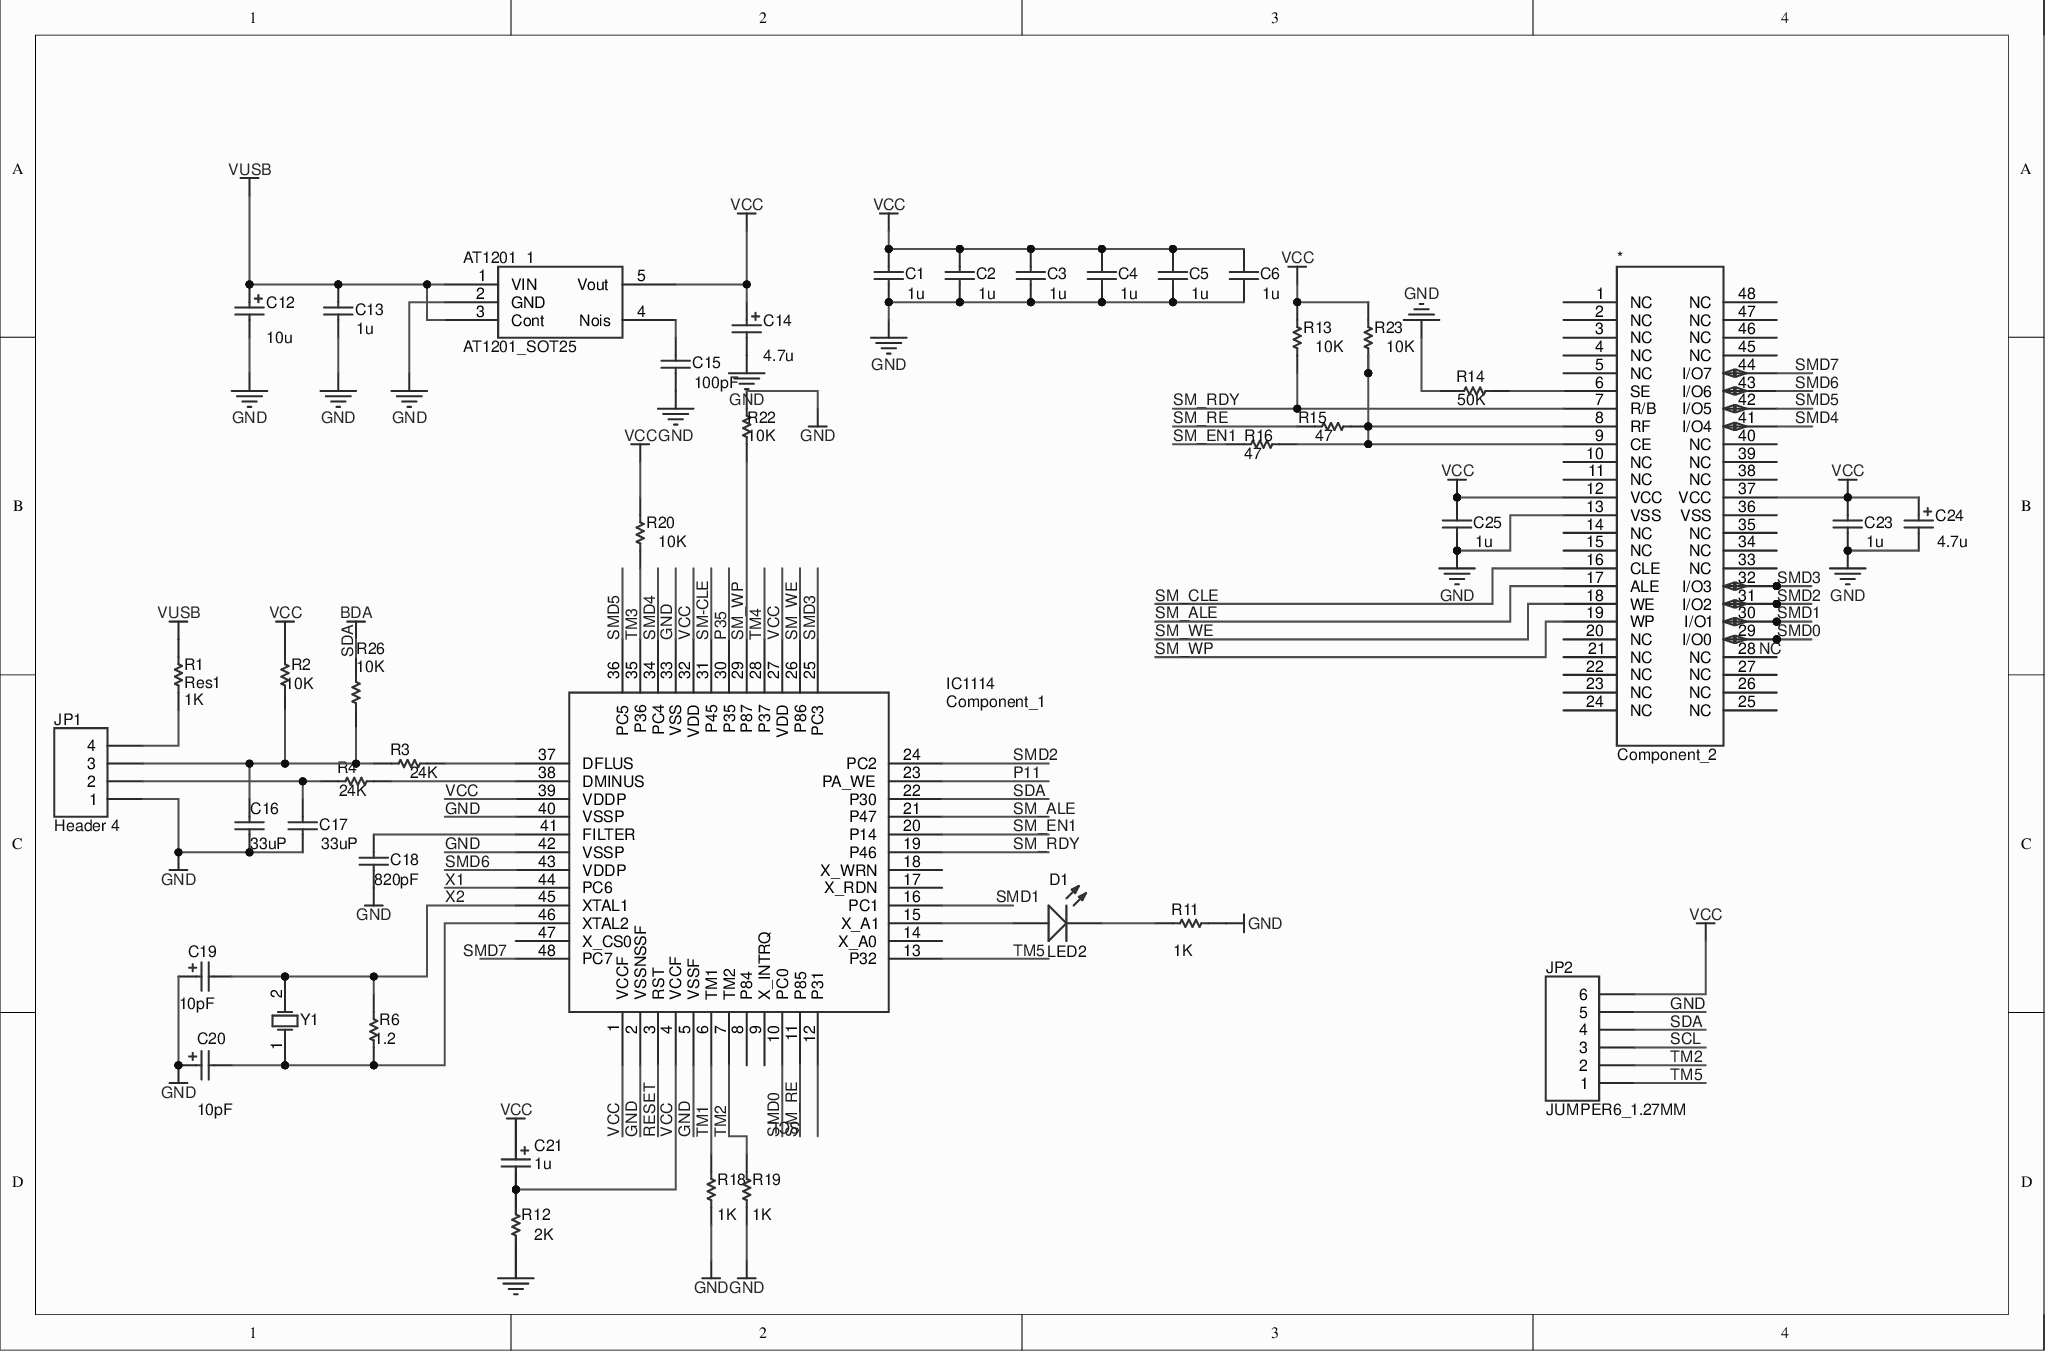
[diagram p0: MISC75231-3.schdoc]
# Altium project MISC75231-2.PrjPcb
1 sheet, 43 parts. Net scope: global (net labels, ports and power ports of the same name join across sheets).
Board file: MISC75231.pcbdoc

## Sheet MISC75231-3.schdoc
size 292 x 193 mm; Name: MISC75231

### Parts
*  Component_2  [DIP48]
AT1201_1  AT1201_SOT25  [SOP6]
C1  value 1u  [RAD-0.3]
C2  value 1u  [RAD-0.3]
C3  value 1u  [RAD-0.3]
C4  value 1u  [RAD-0.3]
C5  value 1u  [RAD-0.3]
C6  value 1u  [RAD-0.3]
C12  value 10u  [POLAR0.8]
C13  value 1u  [RAD-0.3]
C14  value 4.7u  [POLAR0.8]
C15  value 100pF  [RAD-0.3]
C16  value 33uP  [RAD-0.3]
C17  value 33uP  [RAD-0.3]
C18  value 820pF  [RAD-0.3]
C19  value 10pF  [POLAR0.8]
C20  value 10pF  [POLAR0.8]
C21  value 1u  [POLAR0.8]
C23  value 1u  [RAD-0.3]
C24  value 4.7u  [POLAR0.8]
C25  value 1u  [RAD-0.3]
D1  LED2  [3.2X1.6X1.1]
IC1114  Component_1  [Quad48]
JP1  Header 4  [HDR1X4]
JP2  JUMPER6_1.27MM  [HDR1X6]
R1  Res1  value 1K  [AXIAL-0.3]
R2  value 10K  [AXIAL-0.3]
R3  value 24K  [AXIAL-0.3]
R4  value 24K  [AXIAL-0.3]
R6  value 1.2  [AXIAL-0.3]
R11  value 1K  [AXIAL-0.3]
R12  value 2K  [AXIAL-0.3]
R13  value 10K  [AXIAL-0.3]
R14  value 50K  [AXIAL-0.3]
R15  value 47  [AXIAL-0.3]
R16  value 47  [AXIAL-0.3]
R18  value 1K  [AXIAL-0.3]
R19  value 1K  [AXIAL-0.3]
R20  value 10K  [AXIAL-0.3]
R22  value 10K  [AXIAL-0.3]
R23  value 10K  [AXIAL-0.3]
R26  value 10K  [AXIAL-0.3]
Y1  (no value)  [R38]

### Nets
GND: *.13(VSS) AT1201_1.2(GND) C1.1 C2.1 C3.1 C4.1 C5.1 C6.1 C12.2 C13.1 C14.2 C15.1 C16.1 C17.2 C18.1 C19.1 C20.1 C23.1 C24.2 C25.1 IC1114.2(VSSNSSF) IC1114.5(VSSF) IC1114.33(VSS) IC1114.40(VSSP) IC1114.42(VSSP) JP1.1 JP2.5 R11.2 R12.1 R14.2 R18.1 R19.1 R22.2
BDA: IC1114.22(P30) JP2.4 R26.2  [also labelled SDA]
VCC: *.12(VCC) *.37(VCC) AT1201_1.5(Vout) C1.2 C2.2 C3.2 C4.2 C5.2 C6.2 C14.1 C21.1 C21.2 C23.2 C24.1 C25.2 IC1114.1(VCCF) IC1114.4(VCCF) IC1114.27(VDD) IC1114.32(VDD) IC1114.39(VDDP) JP2.6 R2.2 R12.2 R13.2 R20.2 R23.2
VUSB: AT1201_1.1(VIN) AT1201_1.3(Cont) C12.1 C13.2 R1.2
P11: IC1114.23(PA_WE)
P35: IC1114.30(P35)
RESET: IC1114.3(RST)
SCL: IC1114.11(P85) JP2.3 R15.1  [also labelled SM_RE]
SM-CLE: IC1114.31(P45)
SM_ALE: *.17(ALE) IC1114.21(P47)
SM_CLE: *.16(CLE)
SM_EN1: IC1114.20(P14) R16.1
SM_RDY: *.7(R/B) IC1114.19(P46) R13.1
SM_WE: *.18(WE) IC1114.26(P86)
SM_WP: *.19(WP) IC1114.29(P87) R22.1
SMD0: *.29(I/O0) IC1114.10(PC0)
SMD1: *.30(I/O1) IC1114.16(PC1)
SMD2: *.31(I/O2) IC1114.24(PC2)
SMD3: *.32(I/O3) IC1114.25(PC3)
SMD4: *.41(I/O4) IC1114.34(PC4)
SMD5: *.42(I/O5) IC1114.36(PC5)
SMD6: *.43(I/O6) IC1114.43(VDDP)
SMD7: *.44(I/O7)
TM1: IC1114.6(TM1) R18.2
TM2: IC1114.7(TM2) JP2.2 R19.2
TM3: IC1114.35(P36) R20.1
TM4: IC1114.28(P37)
TM5: IC1114.13(P32) JP2.1
X1: IC1114.44(PC6)
X2: C19.2 IC1114.45(XTAL1) R6.2 Y1.2(OSC2)
Net*_6: *.6(SE) R14.1
Net*_8: *.8(RF) *.9(CE) R15.2 R16.2 R23.1
NetAT1201_1_4: AT1201_1.4(Nois) C15.2
NetC16_2: C16.2 JP1.3 R2.1 R3.1 R26.1
NetC17_1: C17.1 JP1.2 R4.1
NetC18_2: C18.2 IC1114.41(FILTER)
NetC20_2: C20.2 IC1114.46(XTAL2) R6.1 Y1.1(OSC1)
NetD1_1: D1.1(A) IC1114.15(X_A1)
NetD1_2: D1.2(K) R11.1
NetIC1114_37: IC1114.37(DFLUS) R3.2
NetIC1114_38: IC1114.38(DMINUS) R4.2
NetJP1_4: JP1.4 R1.1

Not connected (* = marked no-connect by the designer): * 1(NC)* 2(NC)* 3(NC)* 4(NC)* 5(NC)* 10(NC)* 11(NC)* 14(NC) 15(NC)* 20(NC)* 21(NC)* 22(NC)* 23(NC)* 24(NC)* 25(NC)* 26(NC)* 27(NC)* 28(NC)* 33(NC)* 34(NC)* 35(NC)* 36(VSS) 38(NC)* 39(NC)* 40(NC)* 45(NC)* 46(NC)* 47(NC)* 48(NC)*; IC1114 8(P84)* 9(X_INTRQ)* 12(P31) 14(X_A0) 17(X_RDN)* 18(X_WRN)* 47(X_CS0)* 48(PC7)

### Notes on the sheet
- Labels drawn without touching a wire or pin: NC, SMD7

### Library data of the parts
* = Component_2: UniqueId: dc55b09e814ab7ff; AddInBom: yes; Device: Component_2; DesignItemID: Component_2; LibraryName: Schlib1; SymbolName: Component_2; FootprintName: DIP48
AT1201_1 = AT1201_SOT25: UniqueId: a1da92f836eef546; SymbolName: Component_3; AddInBom: yes; Device: AT1201_SOT25; DesignItemID: Component_3; LibraryName: Schlib1; FootprintName: SOP6
C1 = C1: Capacitor; UniqueId: 5fb4f22ffcb6a001; SymbolName: Cap; AddInBom: yes; Device: C1; Published: 8-Jun-2000; LatestRevisionDate: 17-Jul-2002; LatestRevisionNote: Re-released for DXP Platform.; PackageReference: RAD-0.3; PackageDescription: Radial Cap, Thru-Hole; 2 Leads; 0.3 in Pin Spacing; DesignItemID: Cap; LibraryName: Miscellaneous Devices; FootprintName: RAD-0.3; Publisher: Altium Limited
C2 = C2: Capacitor; UniqueId: 21d50210554cb61f; SymbolName: Cap; AddInBom: yes; Device: C2; Published: 8-Jun-2000; LatestRevisionDate: 17-Jul-2002; LatestRevisionNote: Re-released for DXP Platform.; PackageReference: RAD-0.3; PackageDescription: Radial Cap, Thru-Hole; 2 Leads; 0.3 in Pin Spacing; DesignItemID: Cap; LibraryName: Miscellaneous Devices; FootprintName: RAD-0.3; Publisher: Altium Limited
C3 = C3: Capacitor; UniqueId: ec64484c8c07847f; SymbolName: Cap; AddInBom: yes; Device: C3; Published: 8-Jun-2000; LatestRevisionDate: 17-Jul-2002; LatestRevisionNote: Re-released for DXP Platform.; PackageReference: RAD-0.3; PackageDescription: Radial Cap, Thru-Hole; 2 Leads; 0.3 in Pin Spacing; DesignItemID: Cap; LibraryName: Miscellaneous Devices; FootprintName: RAD-0.3; Publisher: Altium Limited
C4 = C4: Capacitor; UniqueId: 623e2bb2442f04df; SymbolName: Cap; AddInBom: yes; Device: C4; Published: 8-Jun-2000; LatestRevisionDate: 17-Jul-2002; LatestRevisionNote: Re-released for DXP Platform.; PackageReference: RAD-0.3; PackageDescription: Radial Cap, Thru-Hole; 2 Leads; 0.3 in Pin Spacing; DesignItemID: Cap; LibraryName: Miscellaneous Devices; FootprintName: RAD-0.3; Publisher: Altium Limited
C5 = C5: Capacitor; UniqueId: 05d417a4d81547fc; SymbolName: Cap; AddInBom: yes; Device: C5; Published: 8-Jun-2000; LatestRevisionDate: 17-Jul-2002; LatestRevisionNote: Re-released for DXP Platform.; PackageReference: RAD-0.3; PackageDescription: Radial Cap, Thru-Hole; 2 Leads; 0.3 in Pin Spacing; DesignItemID: Cap; LibraryName: Miscellaneous Devices; FootprintName: RAD-0.3; Publisher: Altium Limited
C6 = C6: Capacitor; UniqueId: d45ffe04e43665a4; SymbolName: Cap; AddInBom: yes; Device: C6; Published: 8-Jun-2000; LatestRevisionDate: 17-Jul-2002; LatestRevisionNote: Re-released for DXP Platform.; PackageReference: RAD-0.3; PackageDescription: Radial Cap, Thru-Hole; 2 Leads; 0.3 in Pin Spacing; DesignItemID: Cap; LibraryName: Miscellaneous Devices; FootprintName: RAD-0.3; Publisher: Altium Limited
C12 = C12: Polarized Capacitor (Axial); UniqueId: 4eba2014d94c20ef; SymbolName: Cap Pol2; AddInBom: yes; Device: C12; Published: 8-Jun-2000; LatestRevisionDate: 17-Jul-2002; LatestRevisionNote: Re-released for DXP Platform.; PackageReference: POLAR0.8; PackageDescription: Polarized Capacitor; 2 Leads; DesignItemID: Cap Pol2; LibraryName: Miscellaneous Devices; FootprintName: POLAR0.8; Publisher: Altium Limited
C13 = C13: Capacitor; UniqueId: 8d11a04c32f33369; SymbolName: Cap; AddInBom: yes; Device: C13; Published: 8-Jun-2000; LatestRevisionDate: 17-Jul-2002; LatestRevisionNote: Re-released for DXP Platform.; PackageReference: RAD-0.3; PackageDescription: Radial Cap, Thru-Hole; 2 Leads; 0.3 in Pin Spacing; DesignItemID: Cap; LibraryName: Miscellaneous Devices; FootprintName: RAD-0.3; Publisher: Altium Limited
C14 = C14: Polarized Capacitor (Axial); UniqueId: c9f451b8b2c5f180; SymbolName: Cap Pol2; AddInBom: yes; Device: C14; Published: 8-Jun-2000; LatestRevisionDate: 17-Jul-2002; LatestRevisionNote: Re-released for DXP Platform.; PackageReference: POLAR0.8; PackageDescription: Polarized Capacitor; 2 Leads; DesignItemID: Cap Pol2; LibraryName: Miscellaneous Devices; FootprintName: POLAR0.8; Publisher: Altium Limited
C15 = C15: Capacitor; UniqueId: 4a0fa0f8d5a09ecc; SymbolName: Cap; AddInBom: yes; Device: C15; Published: 8-Jun-2000; LatestRevisionDate: 17-Jul-2002; LatestRevisionNote: Re-released for DXP Platform.; PackageReference: RAD-0.3; PackageDescription: Radial Cap, Thru-Hole; 2 Leads; 0.3 in Pin Spacing; DesignItemID: Cap; LibraryName: Miscellaneous Devices; FootprintName: RAD-0.3; Publisher: Altium Limited
C16 = C16: Capacitor; UniqueId: 6992a3033003bbbd; SymbolName: Cap; AddInBom: yes; Device: C16; Published: 8-Jun-2000; LatestRevisionDate: 17-Jul-2002; LatestRevisionNote: Re-released for DXP Platform.; PackageReference: RAD-0.3; PackageDescription: Radial Cap, Thru-Hole; 2 Leads; 0.3 in Pin Spacing; DesignItemID: Cap; LibraryName: Miscellaneous Devices; FootprintName: RAD-0.3; Publisher: Altium Limited
C17 = C17: Capacitor; UniqueId: 5e7964c847a08933; SymbolName: Cap; AddInBom: yes; Device: C17; Published: 8-Jun-2000; LatestRevisionDate: 17-Jul-2002; LatestRevisionNote: Re-released for DXP Platform.; PackageReference: RAD-0.3; PackageDescription: Radial Cap, Thru-Hole; 2 Leads; 0.3 in Pin Spacing; DesignItemID: Cap; LibraryName: Miscellaneous Devices; FootprintName: RAD-0.3; Publisher: Altium Limited
C18 = C18: Capacitor; UniqueId: 9b976857f3e39318; SymbolName: Cap; AddInBom: yes; Device: C18; Published: 8-Jun-2000; LatestRevisionDate: 17-Jul-2002; LatestRevisionNote: Re-released for DXP Platform.; PackageReference: RAD-0.3; PackageDescription: Radial Cap, Thru-Hole; 2 Leads; 0.3 in Pin Spacing; DesignItemID: Cap; LibraryName: Miscellaneous Devices; FootprintName: RAD-0.3; Publisher: Altium Limited
C19 = C19: Polarized Capacitor (Axial); UniqueId: 7dc0401965f49c44; SymbolName: Cap Pol2; AddInBom: yes; Device: C19; Published: 8-Jun-2000; LatestRevisionDate: 17-Jul-2002; LatestRevisionNote: Re-released for DXP Platform.; PackageReference: POLAR0.8; PackageDescription: Polarized Capacitor; 2 Leads; DesignItemID: Cap Pol2; LibraryName: Miscellaneous Devices; FootprintName: POLAR0.8; Publisher: Altium Limited
C20 = C20: Polarized Capacitor (Axial); UniqueId: da3448d2adf90139; SymbolName: Cap Pol2; AddInBom: yes; Device: C20; Published: 8-Jun-2000; LatestRevisionDate: 17-Jul-2002; LatestRevisionNote: Re-released for DXP Platform.; PackageReference: POLAR0.8; PackageDescription: Polarized Capacitor; 2 Leads; DesignItemID: Cap Pol2; LibraryName: Miscellaneous Devices; FootprintName: POLAR0.8; Publisher: Altium Limited
C21 = C21: Polarized Capacitor (Axial); UniqueId: 8b38ef45c1644f88; SymbolName: Cap Pol2; AddInBom: yes; Device: C21; Published: 8-Jun-2000; LatestRevisionDate: 17-Jul-2002; LatestRevisionNote: Re-released for DXP Platform.; PackageReference: POLAR0.8; PackageDescription: Polarized Capacitor; 2 Leads; DesignItemID: Cap Pol2; LibraryName: Miscellaneous Devices; FootprintName: POLAR0.8; Publisher: Altium Limited
C23 = C23: Capacitor; UniqueId: a6f4b5c625a68d3b; SymbolName: Cap; AddInBom: yes; Device: C23; Published: 8-Jun-2000; LatestRevisionDate: 17-Jul-2002; LatestRevisionNote: Re-released for DXP Platform.; PackageReference: RAD-0.3; PackageDescription: Radial Cap, Thru-Hole; 2 Leads; 0.3 in Pin Spacing; DesignItemID: Cap; LibraryName: Miscellaneous Devices; FootprintName: RAD-0.3; Publisher: Altium Limited
C24 = C24: Polarized Capacitor (Axial); UniqueId: 8647aab959e5cc85; SymbolName: Cap Pol2; AddInBom: yes; Device: C24; Published: 8-Jun-2000; LatestRevisionDate: 17-Jul-2002; LatestRevisionNote: Re-released for DXP Platform.; PackageReference: POLAR0.8; PackageDescription: Polarized Capacitor; 2 Leads; DesignItemID: Cap Pol2; LibraryName: Miscellaneous Devices; FootprintName: POLAR0.8; Publisher: Altium Limited
C25 = C25: Capacitor; UniqueId: 67f8b94986dc5590; SymbolName: Cap; AddInBom: yes; Device: C25; Published: 8-Jun-2000; LatestRevisionDate: 17-Jul-2002; LatestRevisionNote: Re-released for DXP Platform.; PackageReference: RAD-0.3; PackageDescription: Radial Cap, Thru-Hole; 2 Leads; 0.3 in Pin Spacing; DesignItemID: Cap; LibraryName: Miscellaneous Devices; FootprintName: RAD-0.3; Publisher: Altium Limited
D1 = LED2: Typical RED, GREEN, YELLOW, AMBER GaAs LED; UniqueId: de80be6c74b1ca94; AddInBom: yes; Device: LED2; Published: 8-Jun-2000; LatestRevisionDate: 17-Jul-2002; LatestRevisionNote: Re-released for DXP Platform.; PackageVersion: Feb-2002; PackageReference: 3.2X1.6X1.1; PackageDescription: SM LED; 2 Flat Leads; DesignItemID: LED2; LibraryName: Miscellaneous Devices; SymbolName: LED2; FootprintName: 3.2X1.6X1.1; Publisher: Altium Limited
IC1114 = Component_1: UniqueId: 168f2036bffe8c68; AddInBom: yes; Device: Component_1; DesignItemID: Component_1; LibraryName: Schlib1; SymbolName: Component_1; FootprintName: Quad48; ConvertToPcb: yes
JP1 = Header 4: Header, 4-Pin; UniqueId: 3f7cd319db4ef0a6; AddInBom: yes; Device: Header 4; LatestRevisionDate: 17-Jul-2002; LatestRevisionNote: Re-released for DXP Platform.; DesignItemID: Header 4; LibraryName: Miscellaneous Connectors; SymbolName: Header 4; FootprintName: HDR1X4; Publisher: Altium Limited
JP2 = JUMPER6_1.27MM: Header, 6-Pin; UniqueId: e68233645d205bf0; SymbolName: Header 6; AddInBom: yes; Device: JUMPER6_1.27MM; LatestRevisionDate: 17-Jul-2002; LatestRevisionNote: Re-released for DXP Platform.; DesignItemID: Header 6; LibraryName: Miscellaneous Connectors; FootprintName: HDR1X6; Publisher: Altium Limited
R1 = Res1: Resistor; UniqueId: 7fed072ae61f3569; AddInBom: yes; Device: Res1; Published: 8-Jun-2000; LatestRevisionDate: 17-Jul-2002; LatestRevisionNote: Re-released for DXP Platform.; PackageReference: AXIAL-0.3; PackageDescription: Axial Device, Thru-Hole; 2 Leads; 0.3 in Pin Spacing; DesignItemID: Res1; LibraryName: Miscellaneous Devices; SymbolName: Res1; FootprintName: AXIAL-0.3; Publisher: Altium Limited
R2 = R2: Resistor; UniqueId: 06442d24ab060343; SymbolName: Res1; AddInBom: yes; Device: R2; Published: 8-Jun-2000; LatestRevisionDate: 17-Jul-2002; LatestRevisionNote: Re-released for DXP Platform.; PackageReference: AXIAL-0.3; PackageDescription: Axial Device, Thru-Hole; 2 Leads; 0.3 in Pin Spacing; DesignItemID: Res1; LibraryName: Miscellaneous Devices; FootprintName: AXIAL-0.3; Publisher: Altium Limited
R3 = R3: Resistor; UniqueId: 6e26aea592918673; SymbolName: Res1; AddInBom: yes; Device: R3; Published: 8-Jun-2000; LatestRevisionDate: 17-Jul-2002; LatestRevisionNote: Re-released for DXP Platform.; PackageReference: AXIAL-0.3; PackageDescription: Axial Device, Thru-Hole; 2 Leads; 0.3 in Pin Spacing; DesignItemID: Res1; LibraryName: Miscellaneous Devices; FootprintName: AXIAL-0.3; Publisher: Altium Limited
R4 = R4: Resistor; UniqueId: 49359f7360e76581; SymbolName: Res1; AddInBom: yes; Device: R4; Published: 8-Jun-2000; LatestRevisionDate: 17-Jul-2002; LatestRevisionNote: Re-released for DXP Platform.; PackageReference: AXIAL-0.3; PackageDescription: Axial Device, Thru-Hole; 2 Leads; 0.3 in Pin Spacing; DesignItemID: Res1; LibraryName: Miscellaneous Devices; FootprintName: AXIAL-0.3; Publisher: Altium Limited
R6 = R6: Resistor; UniqueId: c9a24d22ca7022dc; SymbolName: Res1; AddInBom: yes; Device: R6; Published: 8-Jun-2000; LatestRevisionDate: 17-Jul-2002; LatestRevisionNote: Re-released for DXP Platform.; PackageReference: AXIAL-0.3; PackageDescription: Axial Device, Thru-Hole; 2 Leads; 0.3 in Pin Spacing; DesignItemID: Res1; LibraryName: Miscellaneous Devices; FootprintName: AXIAL-0.3; Publisher: Altium Limited
R11 = R11: Resistor; UniqueId: 069ba0dc55a84bc8; SymbolName: Res1; AddInBom: yes; Device: R11; Published: 8-Jun-2000; LatestRevisionDate: 17-Jul-2002; LatestRevisionNote: Re-released for DXP Platform.; PackageReference: AXIAL-0.3; PackageDescription: Axial Device, Thru-Hole; 2 Leads; 0.3 in Pin Spacing; DesignItemID: Res1; LibraryName: Miscellaneous Devices; FootprintName: AXIAL-0.3; Publisher: Altium Limited
R12 = R12: Resistor; UniqueId: f574a6082c36e6cb; SymbolName: Res1; AddInBom: yes; Device: R12; Published: 8-Jun-2000; LatestRevisionDate: 17-Jul-2002; LatestRevisionNote: Re-released for DXP Platform.; PackageReference: AXIAL-0.3; PackageDescription: Axial Device, Thru-Hole; 2 Leads; 0.3 in Pin Spacing; DesignItemID: Res1; LibraryName: Miscellaneous Devices; FootprintName: AXIAL-0.3; Publisher: Altium Limited
R13 = R13: Resistor; UniqueId: ff7631ddbc1e2fda; SymbolName: Res1; AddInBom: yes; Device: R13; Published: 8-Jun-2000; LatestRevisionDate: 17-Jul-2002; LatestRevisionNote: Re-released for DXP Platform.; PackageReference: AXIAL-0.3; PackageDescription: Axial Device, Thru-Hole; 2 Leads; 0.3 in Pin Spacing; DesignItemID: Res1; LibraryName: Miscellaneous Devices; FootprintName: AXIAL-0.3; Publisher: Altium Limited
R14 = R14: Resistor; UniqueId: d58291ee940aacae; SymbolName: Res1; AddInBom: yes; Device: R14; Published: 8-Jun-2000; LatestRevisionDate: 17-Jul-2002; LatestRevisionNote: Re-released for DXP Platform.; PackageReference: AXIAL-0.3; PackageDescription: Axial Device, Thru-Hole; 2 Leads; 0.3 in Pin Spacing; DesignItemID: Res1; LibraryName: Miscellaneous Devices; FootprintName: AXIAL-0.3; Publisher: Altium Limited
R15 = R15: Resistor; UniqueId: 615753eb74f5e235; SymbolName: Res1; AddInBom: yes; Device: R15; Published: 8-Jun-2000; LatestRevisionDate: 17-Jul-2002; LatestRevisionNote: Re-released for DXP Platform.; PackageReference: AXIAL-0.3; PackageDescription: Axial Device, Thru-Hole; 2 Leads; 0.3 in Pin Spacing; DesignItemID: Res1; LibraryName: Miscellaneous Devices; FootprintName: AXIAL-0.3; Publisher: Altium Limited
R16 = R16: Resistor; UniqueId: 49a4252fe0d0166e; SymbolName: Res1; AddInBom: yes; Device: R16; Published: 8-Jun-2000; LatestRevisionDate: 17-Jul-2002; LatestRevisionNote: Re-released for DXP Platform.; PackageReference: AXIAL-0.3; PackageDescription: Axial Device, Thru-Hole; 2 Leads; 0.3 in Pin Spacing; DesignItemID: Res1; LibraryName: Miscellaneous Devices; FootprintName: AXIAL-0.3; Publisher: Altium Limited
R18 = R18: Resistor; UniqueId: 1bd7cdeea74e381f; SymbolName: Res1; AddInBom: yes; Device: R18; Published: 8-Jun-2000; LatestRevisionDate: 17-Jul-2002; LatestRevisionNote: Re-released for DXP Platform.; PackageReference: AXIAL-0.3; PackageDescription: Axial Device, Thru-Hole; 2 Leads; 0.3 in Pin Spacing; DesignItemID: Res1; LibraryName: Miscellaneous Devices; FootprintName: AXIAL-0.3; Publisher: Altium Limited
R19 = R19: Resistor; UniqueId: 2e979fad964ca14d; SymbolName: Res1; AddInBom: yes; Device: R19; Published: 8-Jun-2000; LatestRevisionDate: 17-Jul-2002; LatestRevisionNote: Re-released for DXP Platform.; PackageReference: AXIAL-0.3; PackageDescription: Axial Device, Thru-Hole; 2 Leads; 0.3 in Pin Spacing; DesignItemID: Res1; LibraryName: Miscellaneous Devices; FootprintName: AXIAL-0.3; Publisher: Altium Limited
R20 = R20: Resistor; UniqueId: 237b6fcbd18a81e0; SymbolName: Res1; AddInBom: yes; Device: R20; Published: 8-Jun-2000; LatestRevisionDate: 17-Jul-2002; LatestRevisionNote: Re-released for DXP Platform.; PackageReference: AXIAL-0.3; PackageDescription: Axial Device, Thru-Hole; 2 Leads; 0.3 in Pin Spacing; DesignItemID: Res1; LibraryName: Miscellaneous Devices; FootprintName: AXIAL-0.3; Publisher: Altium Limited
R22 = R22: Resistor; UniqueId: c805ee3f93c0e373; SymbolName: Res1; AddInBom: yes; Device: R22; Published: 8-Jun-2000; LatestRevisionDate: 17-Jul-2002; LatestRevisionNote: Re-released for DXP Platform.; PackageReference: AXIAL-0.3; PackageDescription: Axial Device, Thru-Hole; 2 Leads; 0.3 in Pin Spacing; DesignItemID: Res1; LibraryName: Miscellaneous Devices; FootprintName: AXIAL-0.3; Publisher: Altium Limited
R23 = R23: Resistor; UniqueId: d677bbbfc70c791c; SymbolName: Res1; AddInBom: yes; Device: R23; Published: 8-Jun-2000; LatestRevisionDate: 17-Jul-2002; LatestRevisionNote: Re-released for DXP Platform.; PackageReference: AXIAL-0.3; PackageDescription: Axial Device, Thru-Hole; 2 Leads; 0.3 in Pin Spacing; DesignItemID: Res1; LibraryName: Miscellaneous Devices; FootprintName: AXIAL-0.3; Publisher: Altium Limited
R26 = R26: Resistor; UniqueId: c4d44f1d54239503; SymbolName: Res1; AddInBom: yes; Device: R26; Published: 8-Jun-2000; LatestRevisionDate: 17-Jul-2002; LatestRevisionNote: Re-released for DXP Platform.; PackageReference: AXIAL-0.3; PackageDescription: Axial Device, Thru-Hole; 2 Leads; 0.3 in Pin Spacing; DesignItemID: Res1; LibraryName: Miscellaneous Devices; FootprintName: AXIAL-0.3; Publisher: Altium Limited
Y1 = Y1: Crystal Oscillator; UniqueId: c44a0eb1f1b20cbd; SymbolName: XTAL; AddInBom: yes; Device: Y1; Published: 8-Jun-2000; LatestRevisionDate: 17-Jul-2002; LatestRevisionNote: Re-released for DXP Platform.; PackageReference: R38; PackageDescription: Crystal, Thru-Hole; 2 Leads; Body 3.1 x 8.2 mm (Dia.xH); DesignItemID: XTAL; LibraryName: Miscellaneous Devices; FootprintName: R38; Publisher: Altium Limited